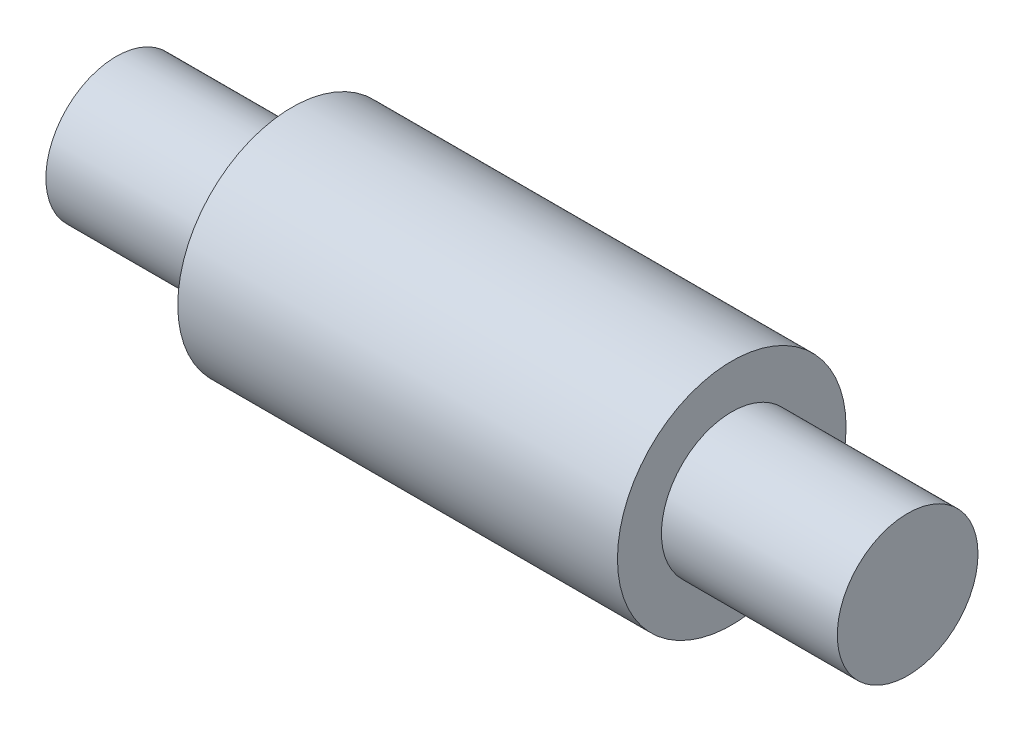
SolidWorks part; units mm, degrees
material "AISI 1045 Steel, cold drawn"
ref_plane "Front Plane" through (0, 0, 0) normal (0, 0, 1) x (1, 0, 0)
ref_plane "Top Plane" through (0, 0, 0) normal (0, 1, 0) x (1, 0, 0)
ref_plane "Right Plane" through (0, 0, 0) normal (1, 0, 0) x (0, 0, -1)
sketch "Sketch1" plane through (0, 0, 0) normal (1, 0, 0) x (0, 0, -1)
  circle A0 centre (0, 0) radius 6.5
  dimension "D1" = 13
extrude "Boss-Extrude1" add sketch "Sketch1" along normal mid plane 25
sketch "Sketch3" plane through (12.5, 0, 0) normal (1, 0, 0) x (0, 0, -1)
  circle A0 centre (0, 0) radius 4
  dimension "D1" = 8
extrude "Boss-Extrude2" add sketch "Sketch3" along normal blind 10
mirror "Mirror1" about plane through (0, 0, 0) normal (1, 0, 0) of "Boss-Extrude2"
